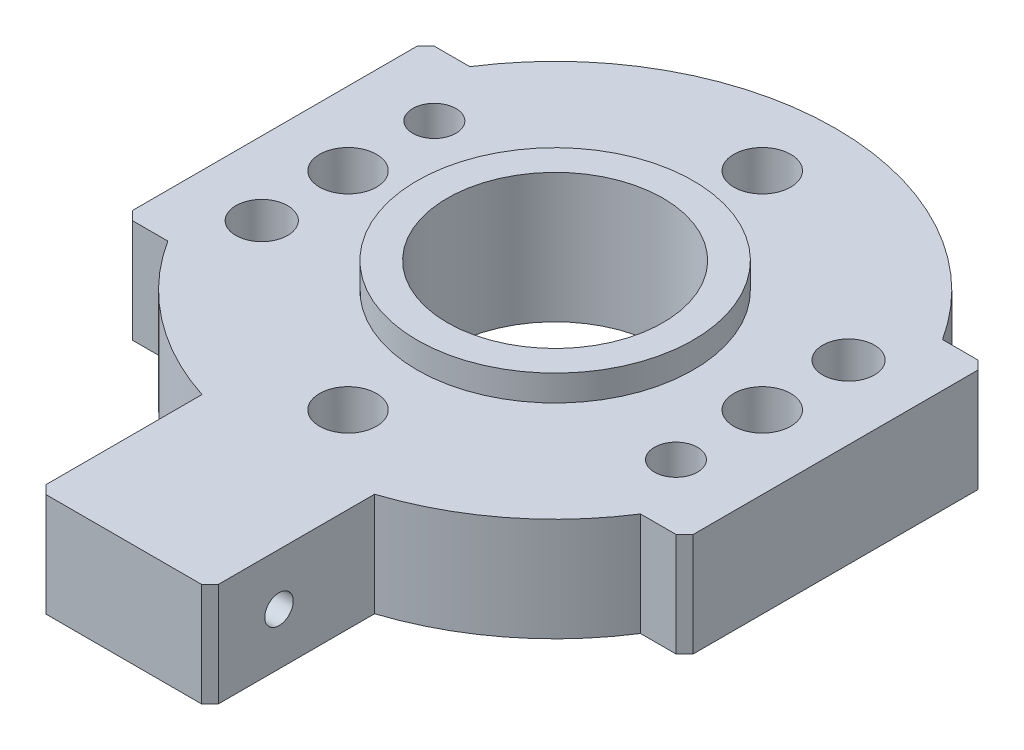
from build123d import *

# Parameters (mm, degrees)
EXTRUDE_1_DEPTH              = 15
SKETCH_2_OUTSIDE_W           = 88.22
SKETCH_2_OUTSIDE_H           = 105.72
SKETCH_2_OUTSIDE_R           = 16
CUT_EXTRUDE_1_DEPTH          = 3
SKETCH_3_R                   = 12.5
CUT_EXTRUDE_2_DEPTH          = 62.491869381
HOLE_WIZARD_M6_1_D           = 6.6
HOLE_WIZARD_M6_1_CBORE_D     = 10
HOLE_WIZARD_M6_1_CBORE_DEPTH = 6.8
F_6_0MM_1_D                  = 6
HOLE_WIZARD_M4_1_D           = 3.3
HOLE_WIZARD_M6_2_D           = 5
CHAMFER_1_SIZE               = 1


with BuildPart() as part:
    # 草图1 → 凸台-拉伸1 (new body)
    with BuildSketch(Plane(origin=(0, 0, 0), x_dir=(1, 0, 0), z_dir=(0, 1, 0))):
        with BuildLine():
            Line((-10, -30.923292192), (-10, -50))
            Line((-10, -50), (10, -50))
            Line((10, -50), (10, -30.923292192))
            ThreePointArc((10, -30.923292192), (19.861440851, -25.724952231), (27.386127875, -17.5))
            Line((27.386127875, -17.5), (32.5, -17.5))
            Line((32.5, -17.5), (32.5, 17.5))
            Line((32.5, 17.5), (27.386127875, 17.5))
            ThreePointArc((27.386127875, 17.5), (0, 32.5), (-27.386127875, 17.5))
            Line((-27.386127875, 17.5), (-32.5, 17.5))
            Line((-32.5, 17.5), (-32.5, -17.5))
            Line((-32.5, -17.5), (-27.386127875, -17.5))
            ThreePointArc((-27.386127875, -17.5), (-19.861440851, -25.724952231), (-10, -30.923292192))
        make_face()
    extrude(amount=EXTRUDE_1_DEPTH)

    # 草图2 outside → 切除-拉伸1 (cut)
    with BuildSketch(Plane(origin=(0, 15, 0), x_dir=(1, 0, 0), z_dir=(0, 1, 0))):
        with Locations((0, -8.75)):
            Rectangle(SKETCH_2_OUTSIDE_W, SKETCH_2_OUTSIDE_H)
        with Locations(Location((0, 0, 0), (0, 0, 270))):
            Circle(SKETCH_2_OUTSIDE_R, mode=Mode.SUBTRACT)
    extrude(amount=-CUT_EXTRUDE_1_DEPTH, mode=Mode.SUBTRACT)

    # 草图3 → 切除-拉伸2 (cut, through all)
    with BuildSketch(Plane.XZ):
        with Locations(Location((0, 0, 0), (0, 0, 270))):
            Circle(SKETCH_3_R)
    extrude(amount=-CUT_EXTRUDE_2_DEPTH, mode=Mode.SUBTRACT)

    # M6 六角圆柱头螺钉的柱形沉头孔1 (through all)
    with Locations(Plane(origin=(0, 0, 0), x_dir=(-1, 0, 0), z_dir=(0, -1, 0))):
        with Locations((0, 24), (24, 0), (0, -24), (-24, 0)):
            CounterBoreHole(HOLE_WIZARD_M6_1_D / 2, HOLE_WIZARD_M6_1_CBORE_D / 2, HOLE_WIZARD_M6_1_CBORE_DEPTH)

    # Ø6.0mm 暗销孔1 (through all)
    with Locations(Plane(origin=(0, 0, 0), x_dir=(-1, 0, 0), z_dir=(0, -1, 0))):
        with Locations((-24, 10), (24, -10)):
            Hole(F_6_0MM_1_D / 2)

    # M4 螺纹孔1 (through all)
    with Locations(Plane.ZY.offset(10)):
        with Locations((42, 6)):
            Hole(HOLE_WIZARD_M4_1_D / 2)

    # M6 螺纹孔2 (through all)
    with Locations(Plane(origin=(0, 0, 0), x_dir=(-1, 0, 0), z_dir=(0, -1, 0))):
        with Locations((24, 10), (-24, -10)):
            Hole(HOLE_WIZARD_M6_2_D / 2)

    # 倒角1
    chamfer_1_edges = [part.edges().sort_by_distance(p)[0] for p in [
        (10, 6, 50),
        (-10, 6, 50),
        (-32.5, 6, 17.5),
        (-32.5, 6, -17.5),
        (32.5, 6, -17.5),
        (32.5, 6, 17.5),
    ]]
    chamfer(chamfer_1_edges, length=CHAMFER_1_SIZE)


solid = part.part
